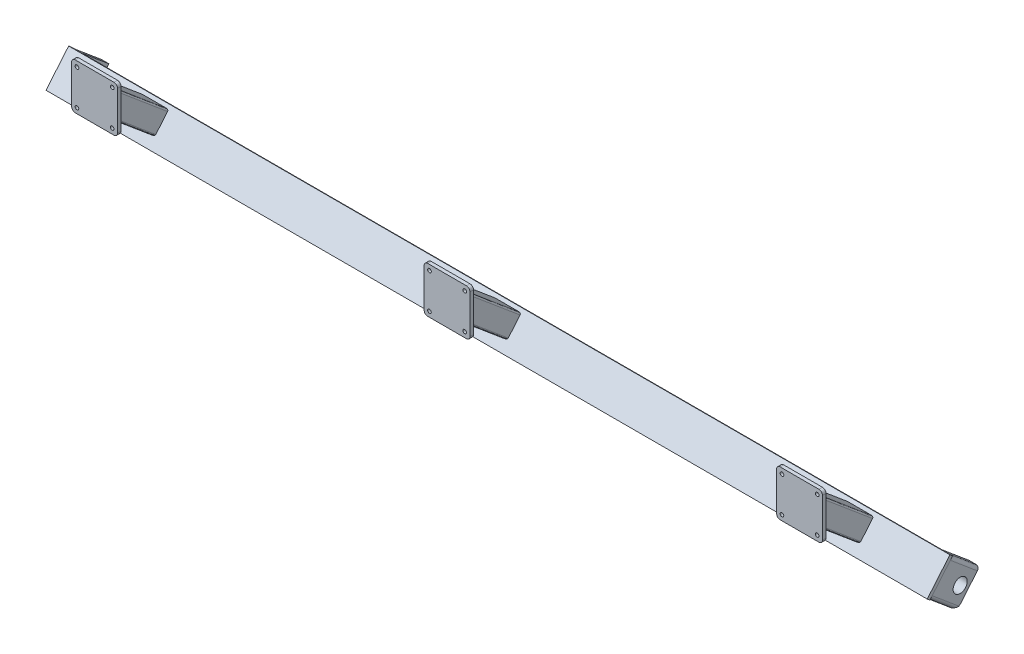
from build123d import *

# Parameters (mm, degrees)
SKETCH_1_R               = 2.6
EXTRUDE_1_DEPTH          = 2.5
CUT_EXTRUDE_1_REACH      = 132.972
SKETCH_6_W               = 1250
SKETCH_6_H               = 50
EXTRUDE_2_DEPTH          = 5
EXTRUDE_3_DEPTH          = 50
EXTRUDE_3_2_DEPTH        = 50
CUT_EXTRUDE_START        = -15
SKETCH_9_R               = 10
CUT_EXTRUDE_2_DEPTH      = 1250
CUT_EXTRUDE_START_2      = -1250
CUT_EXTRUDE_3_DEPTH      = 1250
FILLET_1_R               = 5
FILLET_2_R               = 5
PATTERN_LINEAR_1_COUNT   = 2
PATTERN_LINEAR_1_PITCH   = 500
PATTERN_LINEAR_1_2_COUNT = 2
PATTERN_LINEAR_1_2_PITCH = 500


with BuildPart() as part:
    # 草图1 → 凸台-拉伸1 (new, symmetric)
    with BuildSketch(Plane.XY):
        with BuildLine():
            Line((-27.5, 32.5), (27.5, 32.5))
            ThreePointArc((27.5, 32.5), (31.035533906, 31.035533906), (32.5, 27.5))
            Line((32.5, 27.5), (32.5, -27.5))
            ThreePointArc((32.5, -27.5), (31.035533906, -31.035533906), (27.5, -32.5))
            Line((27.5, -32.5), (-27.5, -32.5))
            ThreePointArc((-27.5, -32.5), (-31.035533906, -31.035533906), (-32.5, -27.5))
            Line((-32.5, -27.5), (-32.5, 27.5))
            ThreePointArc((-32.5, 27.5), (-31.035533906, 31.035533906), (-27.5, 32.5))
        make_face()
        with Locations((-25, 25)):
            Circle(SKETCH_1_R, mode=Mode.SUBTRACT)
        with Locations((25, 25)):
            Circle(SKETCH_1_R, mode=Mode.SUBTRACT)
        with Locations((25, -25)):
            Circle(SKETCH_1_R, mode=Mode.SUBTRACT)
        with Locations((-25, -25)):
            Circle(SKETCH_1_R, mode=Mode.SUBTRACT)
    extrude(amount=EXTRUDE_1_DEPTH, both=True)

    # 扫描1: sweep along a path in 草图2
    with BuildLine(Plane(origin=(0, 0, 0), x_dir=(0, 0, -1), z_dir=(1, 0, 0))) as sweep_1_path:
        Line((2.5, 0), (82.5, -67.127970494))
    # 草图4 → 扫描1 (sweep)
    with BuildSketch(Plane(origin=(0, 0, -2.5), x_dir=(-1, 0, 0), z_dir=(0, 0, -1))):
        with BuildLine():
            Line((17, -20), (-17, -20))
            ThreePointArc((-17, -20), (-19.121320344, -19.121320344), (-20, -17))
            Line((-20, -17), (-20, 17))
            ThreePointArc((-20, 17), (-19.121320344, 19.121320344), (-17, 20))
            Line((-17, 20), (17, 20))
            ThreePointArc((17, 20), (19.121320344, 19.121320344), (20, 17))
            Line((20, 17), (20, -17))
            ThreePointArc((20, -17), (19.121320344, -19.121320344), (17, -20))
        make_face()
        with BuildLine():
            Line((-18, -17), (-18, 17))
            ThreePointArc((-18, 17), (-17.707106781, 17.707106781), (-17, 18))
            Line((-17, 18), (17, 18))
            ThreePointArc((17, 18), (17.707106781, 17.707106781), (18, 17))
            Line((18, 17), (18, -17))
            ThreePointArc((18, -17), (17.707106781, -17.707106781), (17, -18))
            Line((17, -18), (-17, -18))
            ThreePointArc((-17, -18), (-17.707106781, -17.707106781), (-18, -17))
        make_face(mode=Mode.SUBTRACT)
    sweep(path=sweep_1_path.line)

    # 切除-拉伸1: up to this face of the body (flat: up to its plane)
    cut_extrude_1_end = Plane(part.part.faces().sort_by_distance((-20, -33.563985247, -42.5))[0])
    # 草图8 → 切除-拉伸1 (cut, up to the picked face)
    with BuildSketch(Plane(origin=(20, 0, 0), x_dir=(0, 0, -1), z_dir=(1, 0, 0)), mode=Mode.PRIVATE) as cut_extrude_1_sk1:
        Polygon((82.5, -47.127970494), (62.80384494, -70.600934048), (82.5, -87.127970494), (102.576779034, -63.201396953), align=None)
    cut_extrude_1_tool1 = split(extrude(cut_extrude_1_sk1.sketch, amount=-CUT_EXTRUDE_1_REACH, mode=Mode.PRIVATE), bisect_by=cut_extrude_1_end, keep=Keep.BOTH, mode=Mode.PRIVATE)
    add(cut_extrude_1_tool1.solids().sort_by(Axis((20, -67.040567, -82.626875), (-1, 0, 0)))[0], mode=Mode.SUBTRACT)


with BuildPart() as body_2:
    # 草图6 → 凸台-拉伸2 (new body)
    with BuildSketch(Plane(origin=(0, -11.025850582, -112.793275503), x_dir=(-1, 0, 0), z_dir=(0, -0.6427876096865436, -0.7660444431189746))):
        with Locations((0, -67.127970494)):
            Rectangle(SKETCH_6_W, SKETCH_6_H)
    extrude(amount=EXTRUDE_2_DEPTH)


with BuildPart() as body_3:
    # 草图7 → 凸台-拉伸3 (new body)
    with BuildSketch(Plane(origin=(0, -63.309400011, -75.449204908), x_dir=(-1, 0, 0), z_dir=(0, -0.6427876096865436, -0.7660444431189745))):
        with BuildLine():
            Line((-620, 21.927857887), (-610, 21.927857887))
            Line((-610, 21.927857887), (-610, -28.072142113))
            Line((-610, -28.072142113), (-620, -28.072142113))
            ThreePointArc((-620, -28.072142113), (-623.535533906, -26.607676019), (-625, -23.072142113))
            Line((-625, -23.072142113), (-625, 16.927857887))
            ThreePointArc((-625, 16.927857887), (-623.535533906, 20.463391793), (-620, 21.927857887))
        make_face()
    extrude(amount=EXTRUDE_3_DEPTH)


with BuildPart() as body_4:
    # 草图7 → Extrude 3 2 (new body)
    with BuildSketch(Plane(origin=(0, -63.309400011, -75.449204908), x_dir=(-1, 0, 0), z_dir=(0, -0.6427876096865436, -0.7660444431189745))):
        with BuildLine():
            Line((620, 21.927857887), (610, 21.927857887))
            Line((610, 21.927857887), (610, -28.072142113))
            Line((610, -28.072142113), (620, -28.072142113))
            ThreePointArc((620, -28.072142113), (623.535533906, -26.607676019), (625, -23.072142113))
            Line((625, -23.072142113), (625, 16.927857887))
            ThreePointArc((625, 16.927857887), (623.535533906, 20.463391793), (620, 21.927857887))
        make_face()
    extrude(amount=EXTRUDE_3_2_DEPTH)


with BuildPart() as cut_extrude_2_tool:
    # 草图9 → 切除-拉伸2 (new body)
    with BuildSketch(Plane.ZY.offset(-610).offset(CUT_EXTRUDE_START)):
        with Locations(Location((-100.286025531, -88.160363744, 0), (0, 0, 270))):
            Circle(SKETCH_9_R)
    extrude(amount=CUT_EXTRUDE_2_DEPTH)


with BuildPart() as body_3_1:
    add(body_3.part)

    # 切除-拉伸2: cut by cut_extrude_2_tool
    add(cut_extrude_2_tool.part, mode=Mode.SUBTRACT)


with BuildPart() as body_4_1:
    add(body_4.part)

    # 切除-拉伸2: cut by cut_extrude_2_tool
    add(cut_extrude_2_tool.part, mode=Mode.SUBTRACT)


with BuildPart() as cut_extrude_3_tool:
    # 草图10 → 切除-拉伸3 (new body)
    with BuildSketch(Plane(origin=(625, 0, 0), x_dir=(0, 0, -1), z_dir=(1, 0, 0)).offset(CUT_EXTRUDE_START_2)):
        Polygon((98.920939984, -113.123066752), (91.14232085, -113.123066752), (95.707001936, -116.953288967), align=None)
    extrude(amount=CUT_EXTRUDE_3_DEPTH)


with BuildPart() as body_3_2:
    add(body_3_1.part)

    # 切除-拉伸3: cut by cut_extrude_3_tool
    add(cut_extrude_3_tool.part, mode=Mode.SUBTRACT)

    # 圆角1
    fillet_1_edges = [body_3_2.edges().sort_by_distance(p)[0] for p in [
        (617.5, -113.123066752, -98.920939984),
    ]]
    fillet(fillet_1_edges, radius=FILLET_1_R)


with BuildPart() as body_4_2:
    add(body_4_1.part)

    # 切除-拉伸3: cut by cut_extrude_3_tool
    add(cut_extrude_3_tool.part, mode=Mode.SUBTRACT)

    # 圆角2
    fillet_2_edges = [body_4_2.edges().sort_by_distance(p)[0] for p in [
        (-617.5, -113.123066752, -98.920939984),
    ]]
    fillet(fillet_2_edges, radius=FILLET_2_R)


with BuildPart() as pattern_linear_1_1:
    # 阵列(线性)1: pattern copy
    add(part.part.moved(Location(Vector(-1, 0, 0) * (1 * PATTERN_LINEAR_1_PITCH))))


with BuildPart() as pattern_linear_1_2_1:
    # Pattern Linear 1 2: pattern copy
    add(part.part.moved(Location(Vector(1, 0, 0) * (1 * PATTERN_LINEAR_1_2_PITCH))))


solid = Compound([part.part, body_2.part, body_3_2.part, body_4_2.part, pattern_linear_1_1.part, pattern_linear_1_2_1.part])
